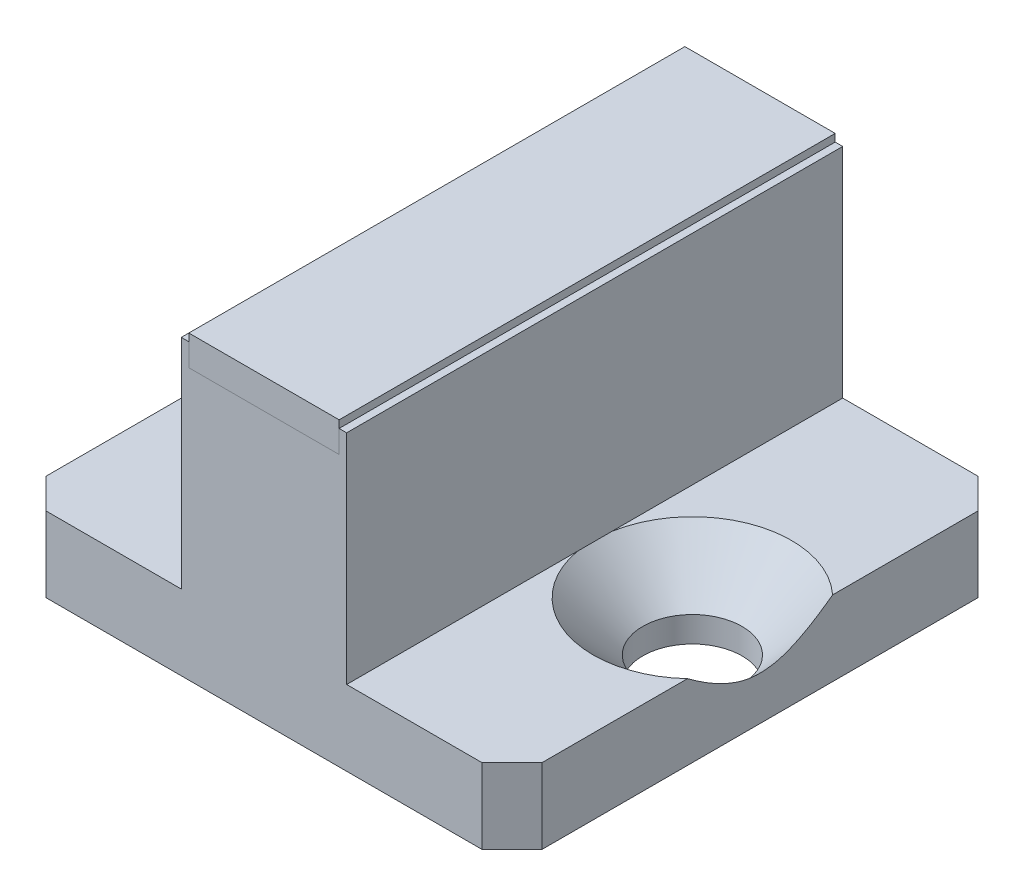
from build123d import *

# Parameters (mm, degrees)
BOSS_EXTRUDE1_DEPTH                          = 16.5
SKETCH2_W                                    = 10
SKETCH2_H                                    = 1.5
CUT_EXTRUDE1_DEPTH                           = 42.73128323
SKETCH3_W                                    = 10
SKETCH3_H                                    = 33
BOSS_EXTRUDE2_DEPTH                          = 2
HOLE_SIZE_PER_CROSS_RECESS_WOOD_SCRE_2_COUNT = 2
HOLE_SIZE_PER_CROSS_RECESS_WOOD_SCRE_2_PITCH = 24
CHAMFER1_SIZE                                = 2


with BuildPart() as part:
    # Sketch1 → Boss-Extrude1 (new, symmetric)
    with BuildSketch(Plane.XY):
        Polygon((16.5, 0), (-16.5, 0), (-16.5, 5), (-5.5, 5), (-5.5, 19.5), (5.5, 19.5), (5.5, 5), (16.5, 5), align=None)
    extrude(amount=BOSS_EXTRUDE1_DEPTH, both=True)

    # Sketch2 → Cut-Extrude1 (cut, through all)
    with BuildSketch(Plane.XY.offset(16.5)):
        with Locations((0, 18.75)):
            Rectangle(SKETCH2_W, SKETCH2_H)
    extrude(amount=-CUT_EXTRUDE1_DEPTH, mode=Mode.SUBTRACT)

    # Sketch4 → Hole size per cross recess wood screw type 1 (revolve, cut)
    with BuildSketch(Plane(origin=(-12, 5, 0), x_dir=(0, 0, 1), z_dir=(1, 0, 0))):
        Polygon((0, 0), (0, 5), (3.3, 5), (3.3, 3.3), (6.6, 0), align=None)
    hole_size_per_cross_recess_wood_screw_ty = revolve(axis=Axis((-12, 11.35, 0), (0, -1, 0)), mode=Mode.SUBTRACT)

    # Hole size per cross recess wood scre 2: Hole size per cross recess wood screw type 1 ×2
    with Locations(*[(i * HOLE_SIZE_PER_CROSS_RECESS_WOOD_SCRE_2_PITCH, 0, 0) for i in range(1, HOLE_SIZE_PER_CROSS_RECESS_WOOD_SCRE_2_COUNT)]):
        add(hole_size_per_cross_recess_wood_screw_ty, mode=Mode.SUBTRACT)

    # Chamfer1
    chamfer1_edges = [part.edges().sort_by_distance(p)[0] for p in [
        (16.5, 2.5, -16.5),
        (-16.5, 2.5, 16.5),
        (16.5, 2.5, 16.5),
        (-16.5, 2.5, -16.5),
    ]]
    chamfer(chamfer1_edges, length=CHAMFER1_SIZE)


with BuildPart() as body_2:
    # Sketch3 → Boss-Extrude2 (new body)
    with BuildSketch(Plane(origin=(0, 18, 0), x_dir=(1, 0, 0), z_dir=(0, 1, 0))):
        Rectangle(SKETCH3_W, SKETCH3_H)
    extrude(amount=BOSS_EXTRUDE2_DEPTH)


solid = Compound([part.part, body_2.part])
